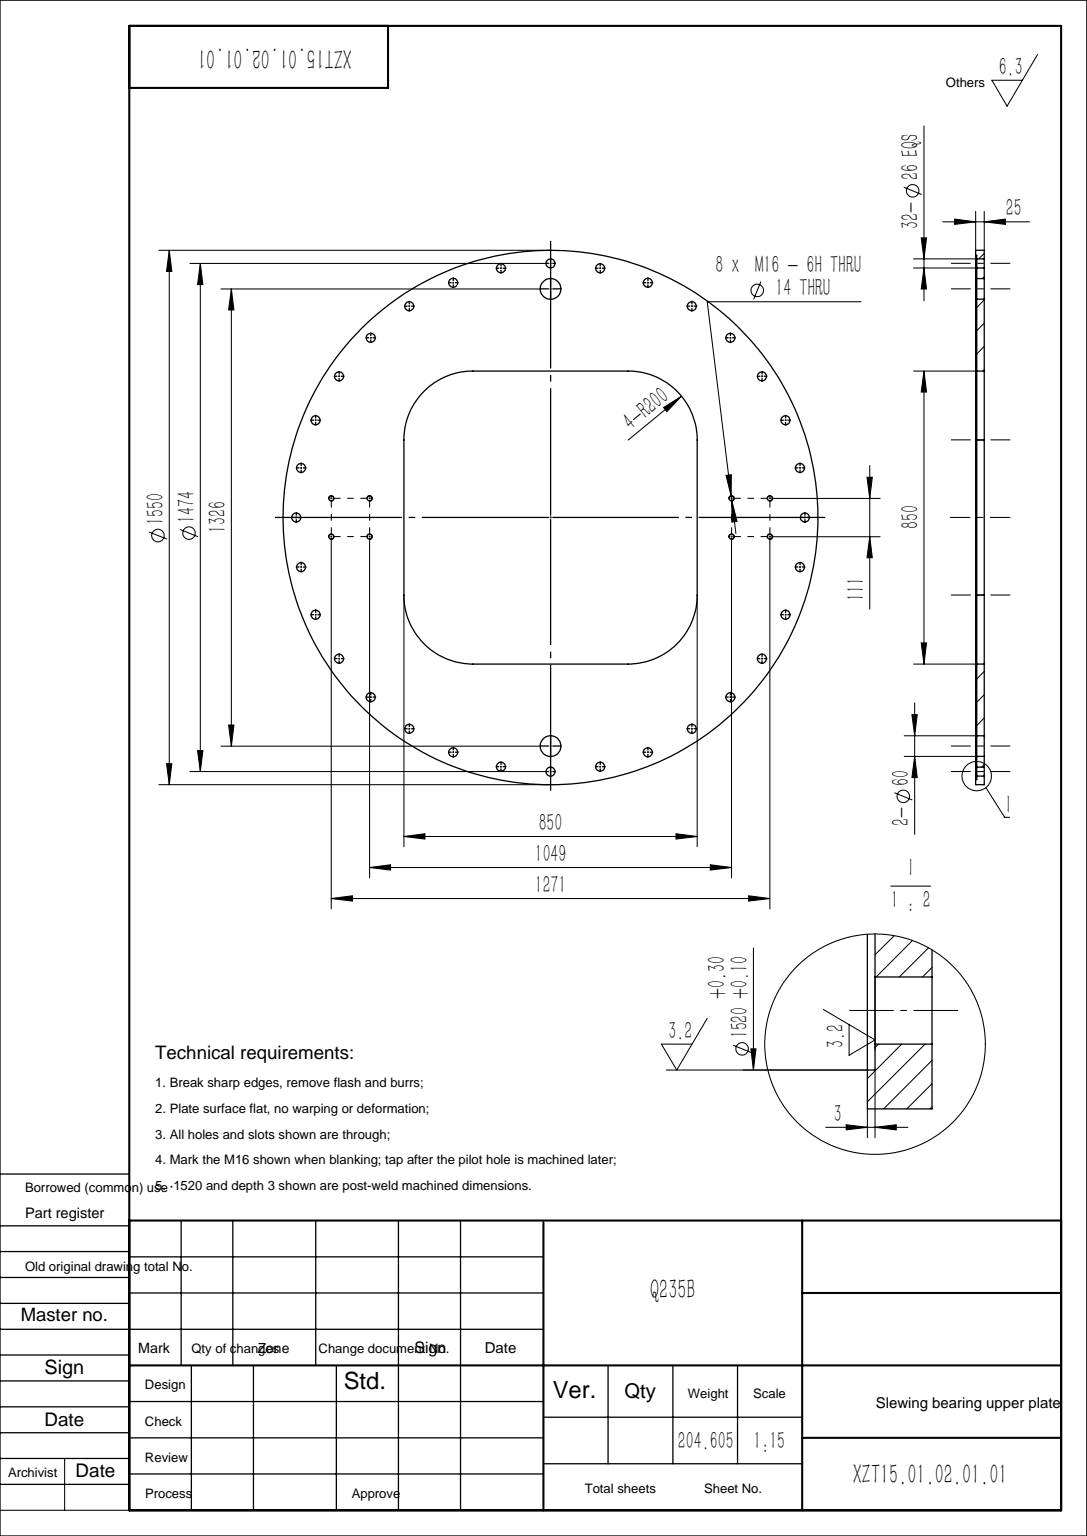
from build123d import *

# Parameters (mm, degrees)
SKETCH1_R           = 775
SKETCH1_R_2         = 30
SKETCH1_R_3         = 13
BOSS_EXTRUDE1_DEPTH = 25
M16_TAPPED_HOLE1_D  = 14
SKETCH4_R           = 760
CUT_EXTRUDE1_DEPTH  = 3


with BuildPart() as part:
    # Sketch1 → Boss-Extrude1 (new body)
    with BuildSketch(Plane(origin=(0, 0, 0), x_dir=(1, 0, 0), z_dir=(0, 1, 0))):
        with Locations(Location((0, 0, 0), (0, 0, 270))):
            Circle(SKETCH1_R)
        with Locations(Location((0, 663, 0), (0, 0, 270))):
            Circle(SKETCH1_R_2, mode=Mode.SUBTRACT)
        with Locations(Location((0, -663, 0), (0, 0, 90))):
            Circle(SKETCH1_R_2, mode=Mode.SUBTRACT)
        with Locations(Location((0, 737, 0), (0, 0, 270))):
            Circle(SKETCH1_R_3, mode=Mode.SUBTRACT)
        with Locations(Location((143.781567326, 722.838751657, 0), (0, 0, 270))):
            Circle(SKETCH1_R_3, mode=Mode.SUBTRACT)
        with Locations(Location((282.037689653, 680.899215461, 0), (0, 0, 270))):
            Circle(SKETCH1_R_3, mode=Mode.SUBTRACT)
        with Locations(Location((409.455261735, 612.793104267, 0), (0, 0, 270))):
            Circle(SKETCH1_R_3, mode=Mode.SUBTRACT)
        with Locations(Location((521.137697734, 521.137697734, 0), (0, 0, 270))):
            Circle(SKETCH1_R_3, mode=Mode.SUBTRACT)
        with Locations(Location((612.793104267, 409.455261735, 0), (0, 0, 270))):
            Circle(SKETCH1_R_3, mode=Mode.SUBTRACT)
        with Locations(Location((680.899215461, 282.037689653, 0), (0, 0, 270))):
            Circle(SKETCH1_R_3, mode=Mode.SUBTRACT)
        with Locations(Location((722.838751657, 143.781567326, 0), (0, 0, 270))):
            Circle(SKETCH1_R_3, mode=Mode.SUBTRACT)
        with Locations(Location((737, 0, 0), (0, 0, 270))):
            Circle(SKETCH1_R_3, mode=Mode.SUBTRACT)
        with Locations(Location((722.838751657, -143.781567326, 0), (0, 0, 270))):
            Circle(SKETCH1_R_3, mode=Mode.SUBTRACT)
        with Locations(Location((680.899215461, -282.037689653, 0), (0, 0, 270))):
            Circle(SKETCH1_R_3, mode=Mode.SUBTRACT)
        with Locations(Location((612.793104267, -409.455261735, 0), (0, 0, 270))):
            Circle(SKETCH1_R_3, mode=Mode.SUBTRACT)
        with Locations(Location((521.137697734, -521.137697734, 0), (0, 0, 270))):
            Circle(SKETCH1_R_3, mode=Mode.SUBTRACT)
        with Locations(Location((409.455261735, -612.793104267, 0), (0, 0, 270))):
            Circle(SKETCH1_R_3, mode=Mode.SUBTRACT)
        with Locations(Location((282.037689653, -680.899215461, 0), (0, 0, 270))):
            Circle(SKETCH1_R_3, mode=Mode.SUBTRACT)
        with Locations(Location((143.781567326, -722.838751657, 0), (0, 0, 270))):
            Circle(SKETCH1_R_3, mode=Mode.SUBTRACT)
        with Locations(Location((0, -737, 0), (0, 0, 270))):
            Circle(SKETCH1_R_3, mode=Mode.SUBTRACT)
        with Locations(Location((-143.781567326, -722.838751657, 0), (0, 0, 270))):
            Circle(SKETCH1_R_3, mode=Mode.SUBTRACT)
        with Locations(Location((-282.037689653, -680.899215461, 0), (0, 0, 270))):
            Circle(SKETCH1_R_3, mode=Mode.SUBTRACT)
        with Locations(Location((-409.455261735, -612.793104267, 0), (0, 0, 270))):
            Circle(SKETCH1_R_3, mode=Mode.SUBTRACT)
        with Locations(Location((-521.137697734, -521.137697734, 0), (0, 0, 270))):
            Circle(SKETCH1_R_3, mode=Mode.SUBTRACT)
        with Locations(Location((-612.793104267, -409.455261735, 0), (0, 0, 270))):
            Circle(SKETCH1_R_3, mode=Mode.SUBTRACT)
        with Locations(Location((-680.899215461, -282.037689653, 0), (0, 0, 270))):
            Circle(SKETCH1_R_3, mode=Mode.SUBTRACT)
        with Locations(Location((-722.838751657, -143.781567326, 0), (0, 0, 270))):
            Circle(SKETCH1_R_3, mode=Mode.SUBTRACT)
        with Locations(Location((-737, 0, 0), (0, 0, 270))):
            Circle(SKETCH1_R_3, mode=Mode.SUBTRACT)
        with Locations(Location((-722.838751657, 143.781567326, 0), (0, 0, 270))):
            Circle(SKETCH1_R_3, mode=Mode.SUBTRACT)
        with Locations(Location((-680.899215461, 282.037689653, 0), (0, 0, 270))):
            Circle(SKETCH1_R_3, mode=Mode.SUBTRACT)
        with Locations(Location((-612.793104267, 409.455261735, 0), (0, 0, 270))):
            Circle(SKETCH1_R_3, mode=Mode.SUBTRACT)
        with Locations(Location((-521.137697734, 521.137697734, 0), (0, 0, 270))):
            Circle(SKETCH1_R_3, mode=Mode.SUBTRACT)
        with Locations(Location((-409.455261735, 612.793104267, 0), (0, 0, 270))):
            Circle(SKETCH1_R_3, mode=Mode.SUBTRACT)
        with Locations(Location((-282.037689653, 680.899215461, 0), (0, 0, 270))):
            Circle(SKETCH1_R_3, mode=Mode.SUBTRACT)
        with Locations(Location((-143.781567326, 722.838751657, 0), (0, 0, 270))):
            Circle(SKETCH1_R_3, mode=Mode.SUBTRACT)
        with BuildLine():
            Line((225, -425), (-225, -425))
            ThreePointArc((-225, -425), (-366.421356237, -366.421356237), (-425, -225))
            Line((-425, -225), (-425, 225))
            ThreePointArc((-425, 225), (-366.421356237, 366.421356237), (-225, 425))
            Line((-225, 425), (225, 425))
            ThreePointArc((225, 425), (366.421356237, 366.421356237), (425, 225))
            Line((425, 225), (425, -225))
            ThreePointArc((425, -225), (366.421356237, -366.421356237), (225, -425))
        make_face(mode=Mode.SUBTRACT)
    extrude(amount=BOSS_EXTRUDE1_DEPTH)

    # M16 Tapped Hole1 (through all)
    with Locations(Plane(origin=(0, 25, 0), x_dir=(1, 0, 0), z_dir=(0, 1, 0))):
        with Locations((-635.5, -55.5), (-524.5, -55.5), (-524.5, 55.5), (-635.5, 55.5), (635.5, 55.5), (524.5, 55.5), (524.5, -55.5), (635.5, -55.5)):
            Hole(M16_TAPPED_HOLE1_D / 2)

    # Sketch4 → Cut-Extrude1 (cut)
    with BuildSketch(Plane.XZ):
        with Locations(Location((0, 0, 0), (0, 0, 270))):
            Circle(SKETCH4_R)
    extrude(amount=-CUT_EXTRUDE1_DEPTH, mode=Mode.SUBTRACT)


solid = part.part
